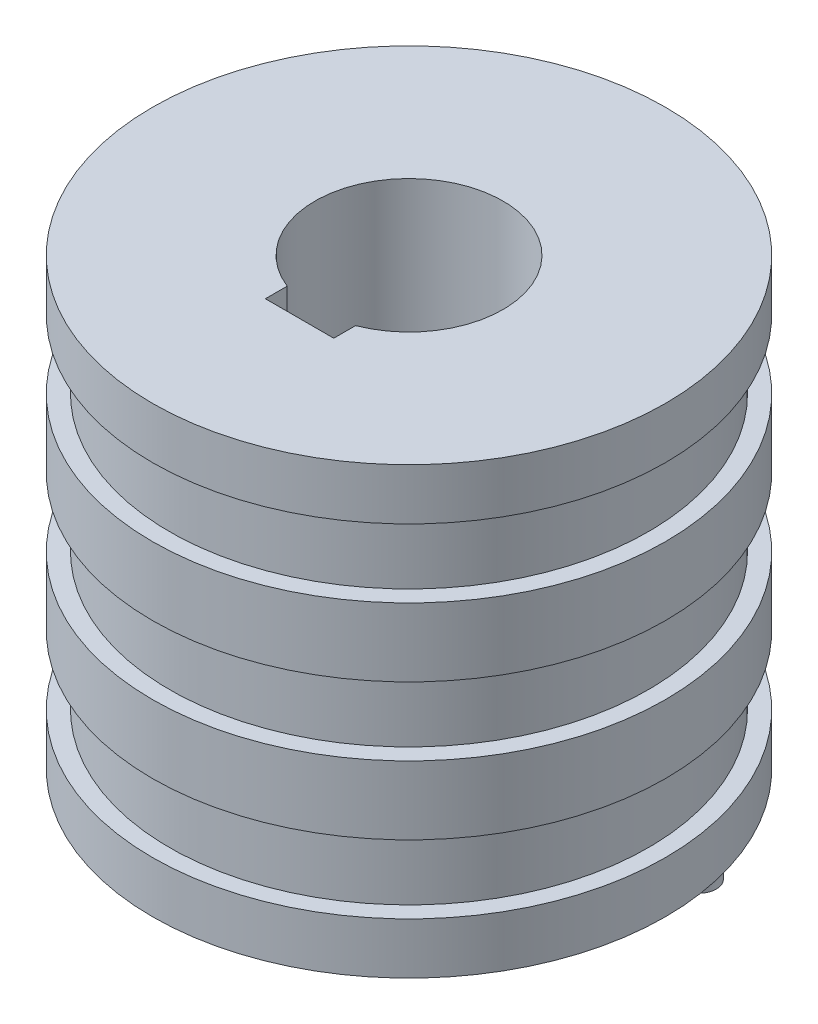
from build123d import *

# Parameters (mm, degrees)
SKETCH3_R           = 27.5
SKETCH3_W           = 20
SKETCH3_H           = 9
CUT_EXTRUDE1_DEPTH  = 130
SKETCH4_R           = 5
BOSS_EXTRUDE3_DEPTH = 28


with BuildPart() as part:
    # Sketch 1 → Revolve1 (revolve)
    with BuildSketch(Plane.XY, mode=Mode.PRIVATE) as revolve1_sk:
        Polygon((70, 75), (75, 75), (75, 95), (70, 95), (70, 115), (75, 115), (75, 130), (0, 130), (0, 0), (75, 0), (75, 15), (70, 15), (70, 35), (75, 35), (75, 55), (70, 55), align=None)
    revolve(revolve1_sk.sketch.rotate(Axis((0, 0, 0), (0, 1, 0)), 90), axis=Axis((0, 0, 0), (0, 1, 0)))

    # Sketch3 → Cut-Extrude1 (cut)
    with BuildSketch(Plane(origin=(0, 130, 0), x_dir=(1, 0, 0), z_dir=(0, 1, 0))):
        Circle(SKETCH3_R)
        with Locations((0, -27.5)):
            Rectangle(SKETCH3_W, SKETCH3_H)
    extrude(amount=-CUT_EXTRUDE1_DEPTH, mode=Mode.SUBTRACT)

    # Sketch4 → Boss-Extrude3 (add)
    with BuildSketch(Plane.XZ):
        with Locations(Location((0, -60, 0), (0, 0, 270))):
            Circle(SKETCH4_R)
        with Locations(Location((42.425, -42.427813696, 0), (0, 0, 270))):
            Circle(SKETCH4_R)
        with Locations(Location((-42.425, -42.427813696, 0), (0, 0, 270))):
            Circle(SKETCH4_R)
    extrude(amount=BOSS_EXTRUDE3_DEPTH)


solid = part.part
